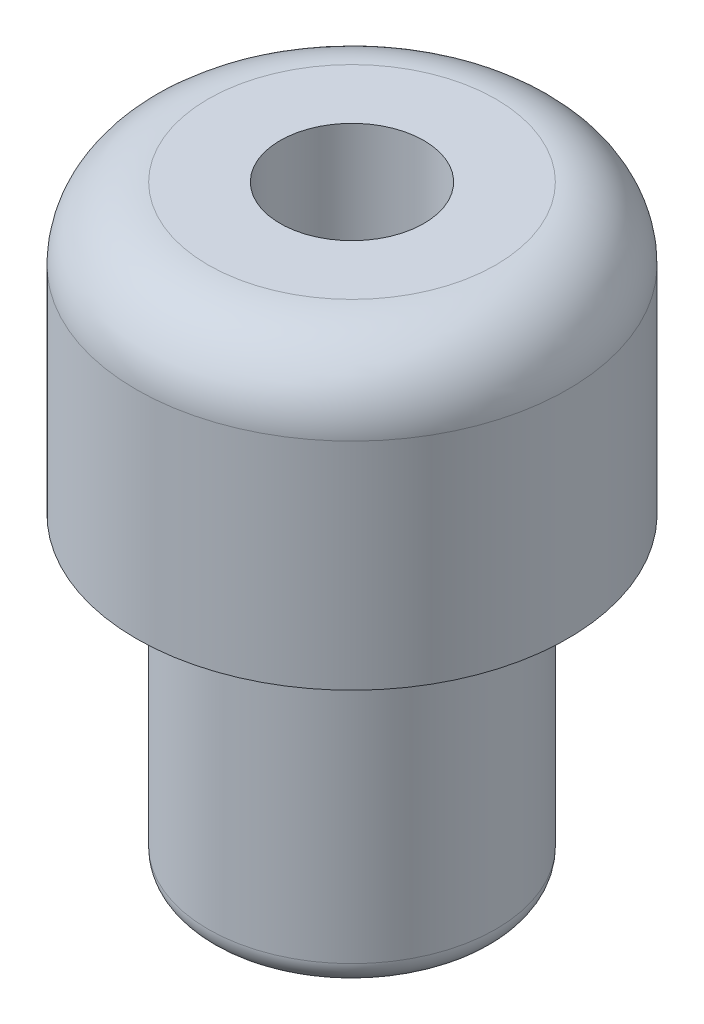
SolidWorks part; units mm, degrees
material "标准件"
ref_plane "前视基准面" through (0, 0, 0) normal (0, 0, 1) x (1, 0, 0)
ref_plane "上视基准面" through (0, 0, 0) normal (0, 1, 0) x (1, 0, 0)
ref_plane "右视基准面" through (0, 0, 0) normal (1, 0, 0) x (0, 0, -1)
sketch "草图1" plane through (0, 0, 0) normal (0, 0, 1) x (1, 0, 0)
  line L0 (0, 0) -> (0, 13.4862) construction
  line L1 (3, 25) -> (3, 0)
  line L2 (3, 0) -> (6, 0)
  line L3 (6, 0) -> (6, 13)
  line L4 (6, 13) -> (9, 13)
  line L5 (9, 13) -> (9, 25)
  line L6 (9, 25) -> (3, 25)
  dimension "D1" = 12
  dimension "D2" = 6
  dimension "D3" = 18
  dimension "D4" = 13
  dimension "D5" = 25
revolve "旋转1" add sketch "草图1" angle 360 about L0
fillet "圆角1" radius 3 1 edges at (0, 25, -9)
fillet "圆角2" radius 1 1 edges at (0, 0, -6)
